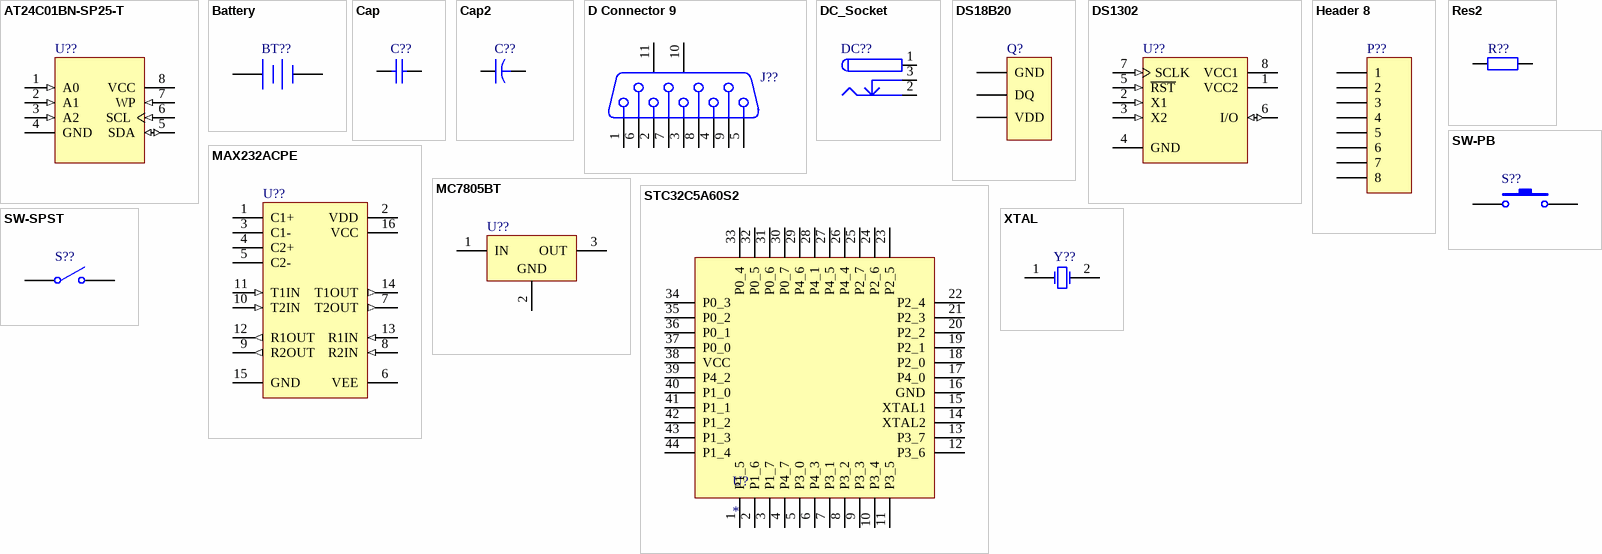
[diagram p0: symbols AT24C01BN-SP25-T to XTAL]
# Altium schematic symbol library MISC84364-3.SCHLIB: 16 symbols
Pins are listed as number, name and electrical type; pins without a type are passive.


## AT24C01BN-SP25-T
designator U??
1Kbit (128 x 8), 2-wire Bus Automotive Serial EEPROM with Write Protect, 2.5V, 8-Pin SOIC, Tape & Reel
footprint 8S1_N (SOIC, 8-Leads, Body 4.9x3.9mm, Pitch 1.27mm, IPC Medium Density)
footprint 8S1_L (SOIC, 8-Leads, Body 4.9x3.9mm, Pitch 1.27mm, IPC High Density)
footprint 8S1_M (SOIC, 8-Leads, Body 4.9x3.9mm, Pitch 1.27mm, IPC Low Density)
pins: 1 A0 (in), 2 A1 (in), 3 A2 (in), 4 GND (power), 5 SDA (io), 6 SCL (in), 7 WP (in), 8 VCC (power)

## Battery
designator BT??
Multicell Battery
footprint BAT-2 (Battery; 2 Leads)
pins: 1 +, 2 -

## Cap
designator C??
Capacitor
footprint RAD-0.3 (Radial Cap, Thru-Hole; 2 Leads; 0.3 in Pin Spacing)
simulation model CAP (Capacitor)
signal-integrity model Cap
footprint RAD-0.1 (Radial Cap, Thru-Hole; 2 Leads; 0.1 in Pin Spacing)
pins: 1, 2

## Cap2
designator C??
Capacitor
footprint CAPR5-4X5 (Capacitor; 2 Leads)
simulation model CAP (Capacitor)
signal-integrity model Cap
pins: 1, 2

## D Connector 9
designator J??
Receptacle Assembly, 9 Position, Right Angle
footprint DSUB1.385-2H9 (Connector; D Subminiature; 9 Position; Right Angle; Pitch 1.385 mm)
signal-integrity model Connector
pins: 1, 2, 3, 4, 5, 6, 7, 8, 9, 10 MH1, 11 MH2

## DC_Socket
designator DC??
footprint DC-002 (3.5X1.1mm)
footprint DC-003 (3.5X1.1mm)
footprint DC-003A (3.5X1.1mm)
footprint DC-005 (5.5X2.1mm)
footprint DC-012 (5.5X2.1mm)
footprint DC-031A (3.5X1.3mm)
footprint DC-050 (5.5X2.1mm)
pins: 1 (power), 2 (power), 3 (power)

## DS18B20
designator Q?
数字温度计
footprint TO92A (92晶体管)
footprint TO92B (92晶体管)
pins: 1 GND, 2 DQ, 3 VDD

## DS1302
designator U??
Trickle Charge Timekeeping Chip
footprint DIP8 (DIP; 8 Leads; Row Spacing 7.62 mm; Pitch 2.54 mm)
pins: 1 VCC2 (power), 2 X1 (in), 3 X2 (in), 4 GND (power), 5 ~{RST} (in), 6 I/O (io), 7 SCLK (in), 8 VCC1 (power)

## Header 8
designator P??
Header, 8-Pin
footprint HDR1X8 (Connector; Header; 8 Position)
signal-integrity model Connector
pins: 1, 2, 3, 4, 5, 6, 7, 8

## MAX232ACPE
designator U??
+5V Powered, Multi-Channel RS-232 Driver/Receiver
footprint PE16A (DIP; 16 Leads; Row Spacing 7.62 mm; Pitch 2.54 mm)
pins: 1 C1+, 2 VDD (power), 3 C1-, 4 C2+, 5 C2-, 6 VEE (power), 7 T2OUT (out), 8 R2IN (in), 9 R2OUT (out), 10 T2IN (in), 11 T1IN (in), 12 R1OUT (out), 13 R1IN (in), 14 T1OUT (out), 15 GND (power), 16 VCC (power)

## MC7805BT
designator U??
3-Terminal Positive Fixed Voltage Regulator
footprint 221A-04 (TO, Thru-Hole, Vertical, Heatsink Mounted; 3 In-Line Leads; Pitch 2.54 mm)
pins: 1 IN (power), 2 GND (power), 3 OUT (power)

## Res2
designator R??
Resistor
footprint AXIAL-0.4 (Axial Device, Thru-Hole; 2 Leads; 0.4 in Pin Spacing)
simulation model RESISTOR (Resistor)
signal-integrity model Res
pins: 1, 2

## STC32C5A60S2
designator U?
STC32C5A60S2
pins: 1 P1_5, 2 P1_6, 3 P1_7, 4 P4_7, 5 P3_0, 6 P4_3, 7 P3_1, 8 P3_2, 9 P3_3, 10 P3_4, 11 P3_5, 12 P3_6, 13 P3_7, 14 XTAL2, 15 XTAL1, 16 GND, 17 P4_0, 18 P2_0, 19 P2_1, 20 P2_2, 21 P2_3, 22 P2_4, 23 P2_5, 24 P2_6, 25 P2_7, 26 P4_4, 27 P4_5, 28 P4_1, 29 P4_6, 30 P0_7, 31 P0_6, 32 P0_5, 33 P0_4, 34 P0_3, 35 P0_2, 36 P0_1, 37 P0_0, 38 VCC, 39 P4_2, 40 P1_0, 41 P1_1, 42 P1_2, 43 P1_3, 44 P1_4

## SW-PB
designator S??
Switch
footprint SPST-2 (Switch; 2 Leads)
pins: 1, 2

## SW-SPST
designator S??
Single-Pole, Single-Throw Switch
footprint SPST-2 (Switch; 2 Leads)
pins: 1 COMMON, 2 NO

## XTAL
designator Y??
Crystal Oscillator
footprint R38 (Crystal, Thru-Hole; 2 Leads; Body 3.1 x 8.2 mm (Dia.xH))
simulation model XTAL (Spice Subcircuit)
pins: 1 OSC1, 2 OSC2